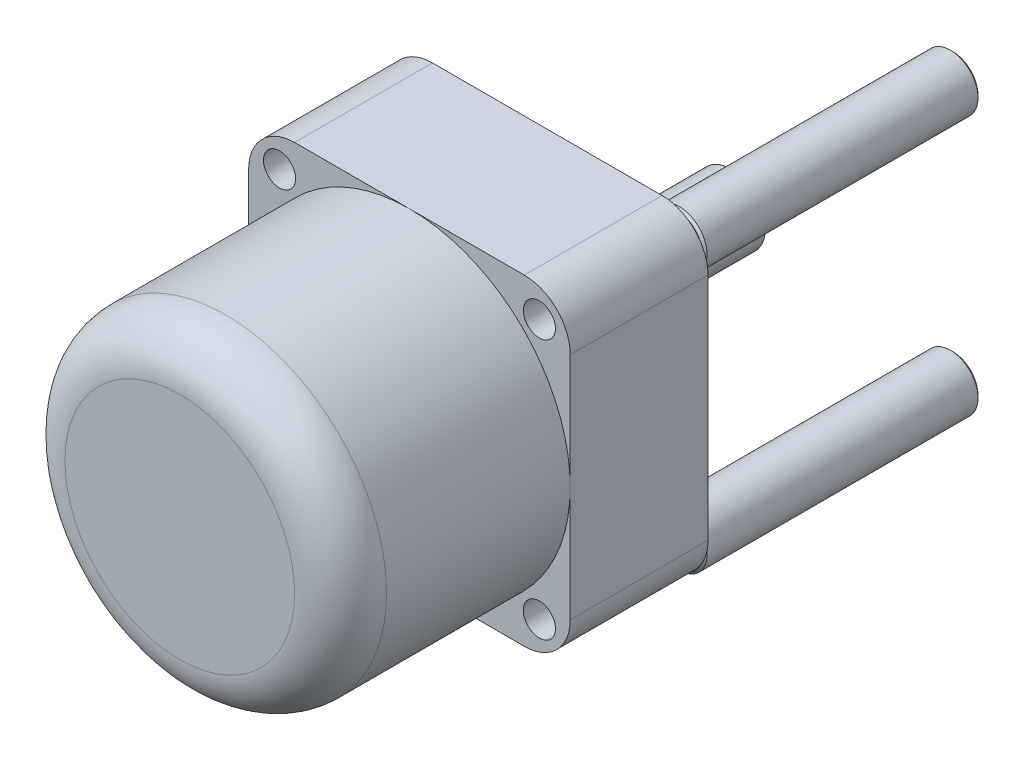
from build123d import *

# Parameters (mm, degrees)
SKETCH1_W                  = 70
SKETCH1_H                  = 70
BOSS_EXTRUDE1_DEPTH        = 30
FILLET2_R                  = 10
SKETCH3_R                  = 3.5
CUT_EXTRUDE1_DEPTH         = 60
SKETCH4_R                  = 22.5
BOSS_EXTRUDE3_DEPTH        = 6
SKETCH5_R                  = 7.5
BOSS_EXTRUDE4_DEPTH        = 35
CHAMFER1_SIZE              = 1
CHAMFER2_SIZE              = 1
CIRPATTERN1_COUNT          = 4
SKETCH6_R                  = 35
BOSS_EXTRUDE5_DEPTH        = 50
FILLET3_R                  = 10
SKETCH7_R                  = 6
BOSS_EXTRUDE6_DEPTH        = 60
BOSS_EXTRUDE6_2_DEPTH      = 60
BOSS_EXTRUDE6_3_DEPTH      = 60
M6_TAPPED_HOLE1_AT_2_COUNT = 2
M6_TAPPED_HOLE1_AT_2_PITCH = 80
M6_TAPPED_HOLE1_AT_3_COUNT = 2
M6_TAPPED_HOLE1_AT_3_PITCH = 56.568542495
CHAMFER3_SIZE              = 0.5
CHAMFER5_SIZE              = 0.5
CHAMFER6_SIZE              = 0.5
M6_TAPPED_HOLE2_AT_2_COUNT = 2
M6_TAPPED_HOLE2_AT_2_PITCH = 80
M6_TAPPED_HOLE2_AT_3_COUNT = 2
M6_TAPPED_HOLE2_AT_3_PITCH = 56.568542495


with BuildPart() as part:
    # Sketch1 → Boss-Extrude1 (new body)
    with BuildSketch(Plane.XY):
        Rectangle(SKETCH1_W, SKETCH1_H)
    extrude(amount=BOSS_EXTRUDE1_DEPTH)

    # Fillet2
    fillet2_edges = [part.edges().sort_by_distance(p)[0] for p in [
        (-35, 35, 15),
        (35, 35, 15),
        (35, -35, 15),
        (-35, -35, 15),
    ]]
    fillet(fillet2_edges, radius=FILLET2_R)

    # Sketch3 → Cut-Extrude1 (cut)
    with BuildSketch(Plane.XY.offset(30)):
        with Locations((-28.284271247, 28.284271247)):
            Circle(SKETCH3_R)
    cut_extrude1 = extrude(amount=-CUT_EXTRUDE1_DEPTH, mode=Mode.SUBTRACT)

    # Sketch4 → Boss-Extrude3 (add)
    with BuildSketch(Plane(origin=(0, 0, 0), x_dir=(-1, 0, 0), z_dir=(0, 0, -1))):
        with Locations(Location((0, 0, 0), (0, 0, 180))):
            Circle(SKETCH4_R)
    extrude(amount=BOSS_EXTRUDE3_DEPTH)

    # Sketch5 → Boss-Extrude4 (add)
    with BuildSketch(Plane(origin=(0, 0, -6), x_dir=(-1, 0, 0), z_dir=(0, 0, -1))):
        Circle(SKETCH5_R)
    extrude(amount=BOSS_EXTRUDE4_DEPTH)

    # Chamfer1
    chamfer1_edges = [part.edges().sort_by_distance(p)[0] for p in [
        (7.5, 0, -41),
    ]]
    chamfer(chamfer1_edges, length=CHAMFER1_SIZE)

    # Chamfer2
    chamfer2_edges = [part.edges().sort_by_distance(p)[0] for p in [
        (-22.5, 0, -6),
    ]]
    chamfer(chamfer2_edges, length=CHAMFER2_SIZE)

    # CirPattern1: Cut-Extrude1 ×4 about axis
    cirpattern1_axis = Axis((0, 0, 0), (0, 0, 1))
    for i in range(1, CIRPATTERN1_COUNT):
        add(cut_extrude1.rotate(cirpattern1_axis, i * 360 / CIRPATTERN1_COUNT), mode=Mode.SUBTRACT)

    # Sketch6 → Boss-Extrude5 (add)
    with BuildSketch(Plane.XY.offset(30)):
        Circle(SKETCH6_R)
    extrude(amount=BOSS_EXTRUDE5_DEPTH)

    # Fillet3
    fillet3_edges = [part.edges().sort_by_distance(p)[0] for p in [
        (-35, 0, 80),
    ]]
    fillet(fillet3_edges, radius=FILLET3_R)


with BuildPart() as body_2:
    # Sketch7 → Boss-Extrude6 (new body)
    with BuildSketch(Plane(origin=(0, 0, 0), x_dir=(-1, 0, 0), z_dir=(0, 0, -1))):
        with Locations((-28.284271247, 28.284271247)):
            Circle(SKETCH7_R)
    extrude(amount=BOSS_EXTRUDE6_DEPTH)

    # Sketch9 → M6 Tapped Hole1 (revolve, cut)
    with BuildSketch(Plane(origin=(28.284271247, 28.284271247, -60), x_dir=(0, 1, 0), z_dir=(1, 0, 0))):
        Polygon((0, 0), (0, 16.502151548), (2.5, 15), (2.5, 0), align=None)
    m6_tapped_hole1 = revolve(axis=Axis((28.284271247, 28.284271247, -66.35), (0, 0, 1)), mode=Mode.SUBTRACT)

    # Chamfer3
    chamfer3_edges = [body_2.edges().sort_by_distance(p)[0] for p in [
        (34.284271247, 28.284271247, 0),
        (34.284271247, 28.284271247, -60),
    ]]
    chamfer(chamfer3_edges, length=CHAMFER3_SIZE)

    # Sketch11 → M6 Tapped Hole2 (revolve, cut)
    with BuildSketch(Plane(origin=(28.284271247, 28.284271247, 0), x_dir=(0, -1, 0), z_dir=(1, 0, 0))):
        Polygon((0, 0), (0, 16.502151548), (2.5, 15), (2.5, 0), align=None)
    m6_tapped_hole2 = revolve(axis=Axis((28.284271247, 28.284271247, 6.35), (0, 0, -1)), mode=Mode.SUBTRACT)


with BuildPart() as body_3:
    # Sketch7 → Boss-Extrude6 2 (new body)
    with BuildSketch(Plane(origin=(0, 0, 0), x_dir=(-1, 0, 0), z_dir=(0, 0, -1))):
        with Locations((28.284271247, -28.284271247)):
            Circle(SKETCH7_R)
    extrude(amount=BOSS_EXTRUDE6_2_DEPTH)

    # M6 Tapped Hole1 at 2: M6 Tapped Hole1 ×2
    with Locations(*[Vector(-0.7071067811865429, -0.7071067811865522, 0) * (i * M6_TAPPED_HOLE1_AT_2_PITCH) for i in range(1, M6_TAPPED_HOLE1_AT_2_COUNT)]):
        add(m6_tapped_hole1, mode=Mode.SUBTRACT)

    # Chamfer6
    chamfer6_edges = [body_3.edges().sort_by_distance(p)[0] for p in [
        (-22.284271247, -28.284271247, 0),
        (-22.284271247, -28.284271247, -60),
    ]]
    chamfer(chamfer6_edges, length=CHAMFER6_SIZE)

    # M6 Tapped Hole2 at 2: M6 Tapped Hole2 ×2
    with Locations(*[Vector(-0.7071067811865429, -0.7071067811865522, 0) * (i * M6_TAPPED_HOLE2_AT_2_PITCH) for i in range(1, M6_TAPPED_HOLE2_AT_2_COUNT)]):
        add(m6_tapped_hole2, mode=Mode.SUBTRACT)


with BuildPart() as body_4:
    # Sketch7 → Boss-Extrude6 3 (new body)
    with BuildSketch(Plane(origin=(0, 0, 0), x_dir=(-1, 0, 0), z_dir=(0, 0, -1))):
        with Locations((-28.284271247, -28.284271247)):
            Circle(SKETCH7_R)
    extrude(amount=BOSS_EXTRUDE6_3_DEPTH)

    # M6 Tapped Hole1 at 3: M6 Tapped Hole1 ×2
    with Locations(*[(0, -i * M6_TAPPED_HOLE1_AT_3_PITCH, 0) for i in range(1, M6_TAPPED_HOLE1_AT_3_COUNT)]):
        add(m6_tapped_hole1, mode=Mode.SUBTRACT)

    # Chamfer5
    chamfer5_edges = [body_4.edges().sort_by_distance(p)[0] for p in [
        (34.284271247, -28.284271247, 0),
        (34.284271247, -28.284271247, -60),
        (28.284271247, -30.784271247, -60),
    ]]
    chamfer(chamfer5_edges, length=CHAMFER5_SIZE)

    # M6 Tapped Hole2 at 3: M6 Tapped Hole2 ×2
    with Locations(*[(0, -i * M6_TAPPED_HOLE2_AT_3_PITCH, 0) for i in range(1, M6_TAPPED_HOLE2_AT_3_COUNT)]):
        add(m6_tapped_hole2, mode=Mode.SUBTRACT)


solid = Compound([part.part, body_2.part, body_3.part, body_4.part])
